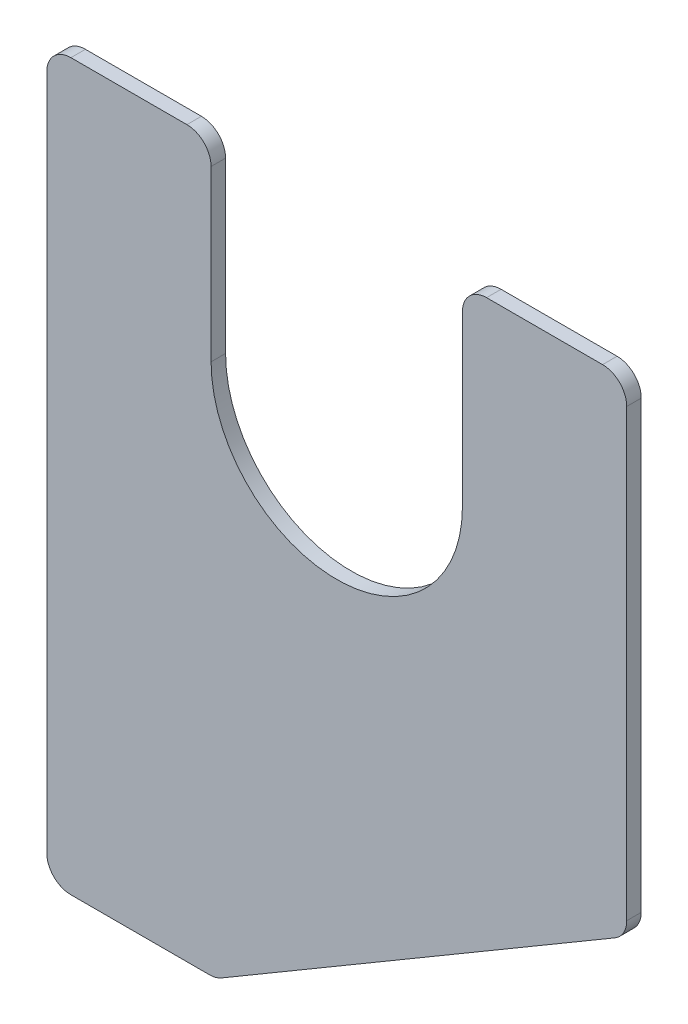
SolidWorks part; units mm, degrees
material "201 退火不锈钢 (SS)"
ref_plane "Front Plane" through (0, 0, 0) normal (0, 0, 1) x (1, 0, 0)
ref_plane "Top Plane" through (0, 0, 0) normal (0, 1, 0) x (1, 0, 0)
ref_plane "Right Plane" through (0, 0, 0) normal (1, 0, 0) x (0, 0, -1)
sketch "Sketch1" plane through (0, 0, 0) normal (0, 0, 1) x (1, 0, 0)
  line L0 (0, -5) -> (0, -145)
  line L1 (5, -150) -> (33.6385, -150)
  line L2 (36.1736, -149.3097) -> (117.5351, -101.4499)
  line L3 (120, -97.1403) -> (120, -5)
  line L5 (5, 0) -> (29, 0)
  line L6 (34, -5) -> (34, -40)
  line L7 (115, 0) -> (91, 0)
  line L8 (86, -5) -> (86, -40)
  line L9 (34, -40) -> (86, -40) construction
  arc A0 (34, -40) -> (86, -40) centre (60, -40) ccw
  arc A1 (91, 0) -> (86, -5) centre (91, -5) ccw
  arc A2 (115, 0) -> (120, -5) centre (115, -5) cw
  arc A3 (120, -97.1403) -> (117.5351, -101.4499) centre (115, -97.1403) cw
  arc A4 (36.1736, -149.3097) -> (33.6385, -150) centre (33.6385, -145) cw
  arc A5 (5, -150) -> (0, -145) centre (5, -145) cw
  arc A6 (34, -5) -> (29, 0) centre (29, -5) ccw
  arc A7 (0, -5) -> (5, 0) centre (5, -5) cw
  point P14 (86, 0)
  point P17 (120, 0)
  point P20 (120, -100)
  point P23 (35, -150)
  point P26 (0, -150)
  point P29 (34, 0)
  point P32 (0, 0)
  dimension "D6" = 52
  dimension "D8" = 5
  dimension "D1" = 150
  dimension "D2" = 35
  dimension "D3" = 120
  dimension "D4" = 100
  dimension "D5" = 40
  dimension "D7" = 34
extrude "Boss-Extrude1" add sketch "Sketch1" along normal blind 3
